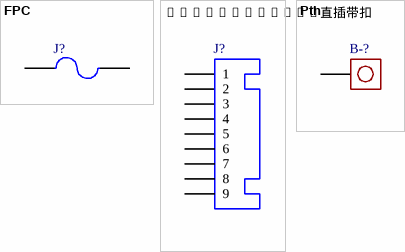
[diagram p0: symbols FPC to Pth]
# Altium schematic symbol library MISC89348.SCHLIB: 3 symbols
Pins are listed as number, name and electrical type; pins without a type are passive.


## FPC
designator J?
footprint 异形电阻
pins: 1, 2

## HX-2.54mm-9P直插带扣
designator J?
HX-2.54mm-9P through-hole connector with latch
footprint HX2.54-5P直插不带扣 (HX2.54-5P through-hole, no latch)
footprint HX2.0-9P
pins: 1, 2, 3, 4, 5, 6, 7, 8, 9

## Pth
designator B-?
Through-hole pad
footprint 4*3 (Through-hole pad)
footprint 35*7*0.3mm
footprint 10*8*0.3mm (Nickel sheet)
footprint 30*6*0.5mm
footprint 55*10*1MM
footprint 55*10*1MM
pins: 1